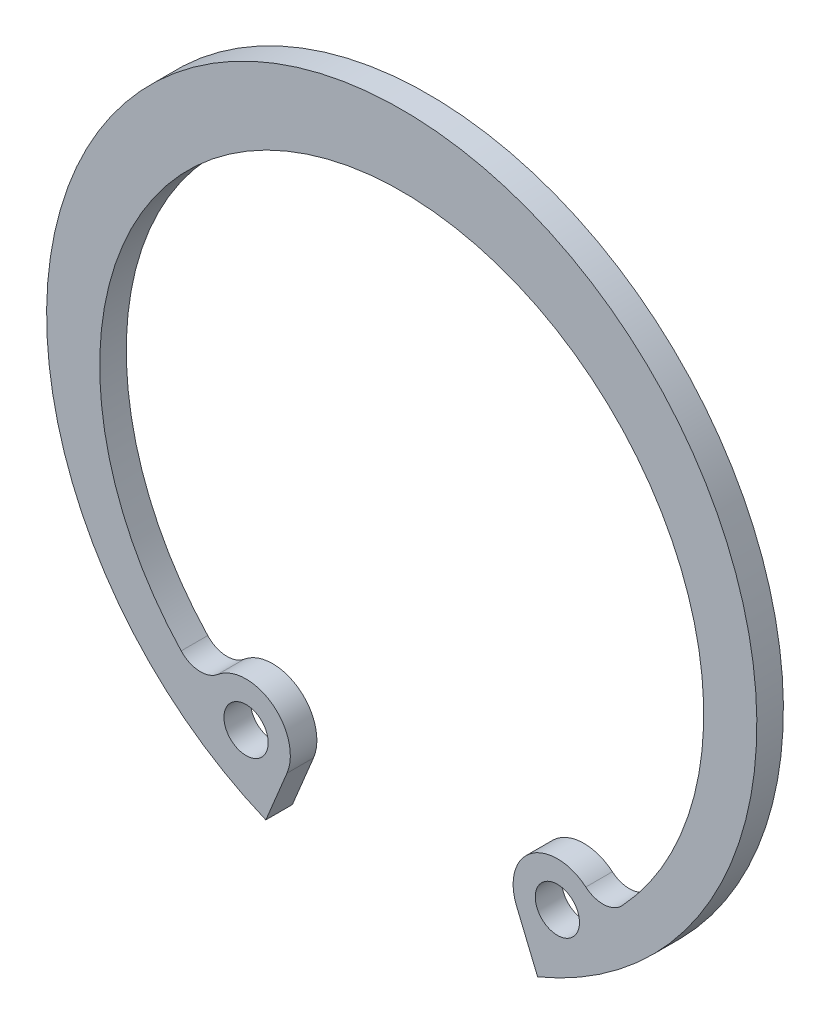
from build123d import *

# Parameters (mm, degrees)
SKETCH1_R  = 1
BODY_DEPTH = 1.2


with BuildPart() as part:
    # Sketch1 → Body (new body)
    with BuildSketch(Plane.XY):
        with BuildLine():
            Line((5.186595963, -12.521550316), (6.142069089, -14.828266497))
            ThreePointArc((6.142069089, -14.828266497), (0, 16.05), (-6.142069089, -14.828266497))
            Line((-6.142069089, -14.828266497), (-5.186595963, -12.521550316))
            ThreePointArc((-5.186595963, -12.521550316), (-5.851927185, -10.143153881), (-8.32029392, -10.224399796))
            ThreePointArc((-8.32029392, -10.224399796), (-9.164022184, -10.503157731), (-9.968180846, -10.125120408))
            ThreePointArc((-9.968180846, -10.125120408), (0, 12.85), (9.968180846, -10.125120408))
            ThreePointArc((9.968180846, -10.125120408), (9.164022184, -10.503157731), (8.32029392, -10.224399796))
            ThreePointArc((8.32029392, -10.224399796), (5.851927185, -10.143153881), (5.186595963, -12.521550316))
        make_face()
        with Locations(Location((7.034355028, -11.756183451, 0), (0, 0, 180))):
            Circle(SKETCH1_R, mode=Mode.SUBTRACT)
        with Locations((-7.034355028, -11.756183451)):
            Circle(SKETCH1_R, mode=Mode.SUBTRACT)
    extrude(amount=-BODY_DEPTH)


solid = part.part
